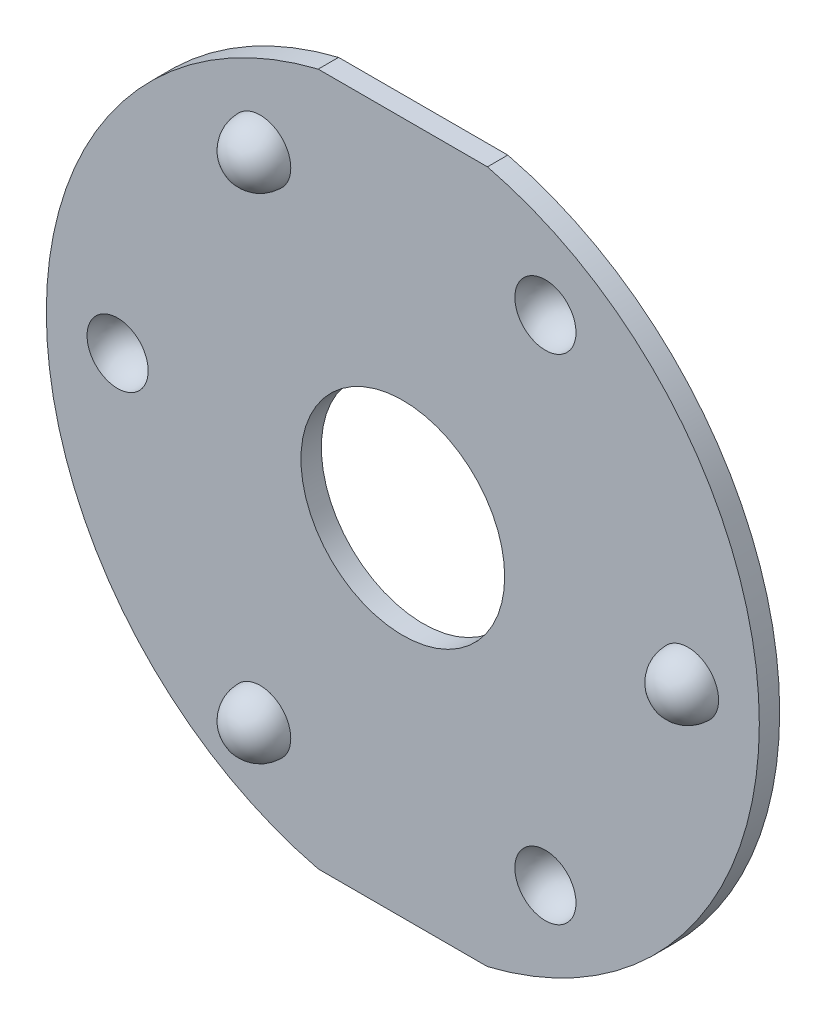
from build123d import *

# Parameters (mm, degrees)
SKETCH1_R           = 17.5
SKETCH1_R_2         = 5
BOSS_EXTRUDE1_DEPTH = 0.5
SKETCH2_W           = 25.230878588
SKETCH2_H           = 11.302160125
SKETCH2_H_2         = 10.824604063
CUT_EXTRUDE1_DEPTH  = 1
CIRPATTERN1_COUNT   = 3
CIRPATTERN2_COUNT   = 3
CIRPATTERN3_COUNT   = 3
CIRPATTERN4_COUNT   = 3


with BuildPart() as part:
    # Sketch1 → Boss-Extrude1 (new, symmetric)
    with BuildSketch(Plane.XY):
        Circle(SKETCH1_R)
        Circle(SKETCH1_R_2, mode=Mode.SUBTRACT)
    extrude(amount=BOSS_EXTRUDE1_DEPTH, both=True)

    # Sketch2 → Cut-Extrude1 (cut)
    with BuildSketch(Plane.XY.offset(0.5)):
        with Locations((0, 22.651080063)):
            Rectangle(SKETCH2_W, SKETCH2_H)
        with Locations((0, -22.412302032)):
            Rectangle(SKETCH2_W, SKETCH2_H_2)
    extrude(amount=-CUT_EXTRUDE1_DEPTH, mode=Mode.SUBTRACT)

    # Sketch3 → Revolve1 (revolve)
    with BuildSketch(Plane.XY.offset(0.5)):
        with BuildLine():
            Line((14, 1.5), (14, -1.5))
            ThreePointArc((14, -1.5), (15.5, 0), (14, 1.5))
        make_face()
    revolve1 = revolve(axis=Axis((14, 1.5, 0.5), (0, -1, 0)))

    # CirPattern1: Revolve1 ×3 about axis
    cirpattern1_axis = Axis((0, 0, 0), (0, 0, 1))
    for i in range(1, CIRPATTERN1_COUNT):
        add(revolve1.rotate(cirpattern1_axis, i * 360 / CIRPATTERN1_COUNT))

    # Sketch5 → Revolve2 (revolve)
    with BuildSketch(Plane(origin=(0, 0, -0.5), x_dir=(-1, 0, 0), z_dir=(0, 0, -1))):
        with BuildLine():
            Line((14, -1.5), (14, 1.5))
            ThreePointArc((14, 1.5), (15.5, 0), (14, -1.5))
        make_face()
    revolve2 = revolve(axis=Axis((-14, -1.5, -0.5), (0, 1, 0)))

    # CirPattern2: Revolve2 ×3 about axis
    cirpattern2_axis = Axis((0, 0, 0), (0, 0, 1))
    for i in range(1, CIRPATTERN2_COUNT):
        add(revolve2.rotate(cirpattern2_axis, i * 360 / CIRPATTERN2_COUNT))

    # Sketch6 → Cut-Revolve2 (revolve, cut)
    with BuildSketch(Plane.XY.offset(0.5)):
        with BuildLine():
            Line((-14, 1.5), (-14, -1.5))
            ThreePointArc((-14, -1.5), (-15.5, 0), (-14, 1.5))
        make_face()
    cut_revolve2 = revolve(axis=Axis((-14, 1.5, 0.5), (0, -1, 0)), mode=Mode.SUBTRACT)

    # CirPattern3: Cut-Revolve2 ×3 about axis
    cirpattern3_axis = Axis((0, 0, 0), (0, 0, 1))
    for i in range(1, CIRPATTERN3_COUNT):
        add(cut_revolve2.rotate(cirpattern3_axis, i * 360 / CIRPATTERN3_COUNT), mode=Mode.SUBTRACT)

    # Sketch7 → Cut-Revolve3 (revolve, cut)
    with BuildSketch(Plane(origin=(0, 0, -0.5), x_dir=(-1, 0, 0), z_dir=(0, 0, -1))):
        with BuildLine():
            Line((-14, -1.118033989), (-14, 1.118033989))
            ThreePointArc((-14, 1.118033989), (-15.118033989, 0), (-14, -1.118033989))
        make_face()
    cut_revolve3 = revolve(axis=Axis((14, -1.118033989, -0.5), (0, 1, 0)), mode=Mode.SUBTRACT)

    # CirPattern4: Cut-Revolve3 ×3 about axis
    cirpattern4_axis = Axis((0, 0, 0), (0, 0, 1))
    for i in range(1, CIRPATTERN4_COUNT):
        add(cut_revolve3.rotate(cirpattern4_axis, i * 360 / CIRPATTERN4_COUNT), mode=Mode.SUBTRACT)


solid = part.part
